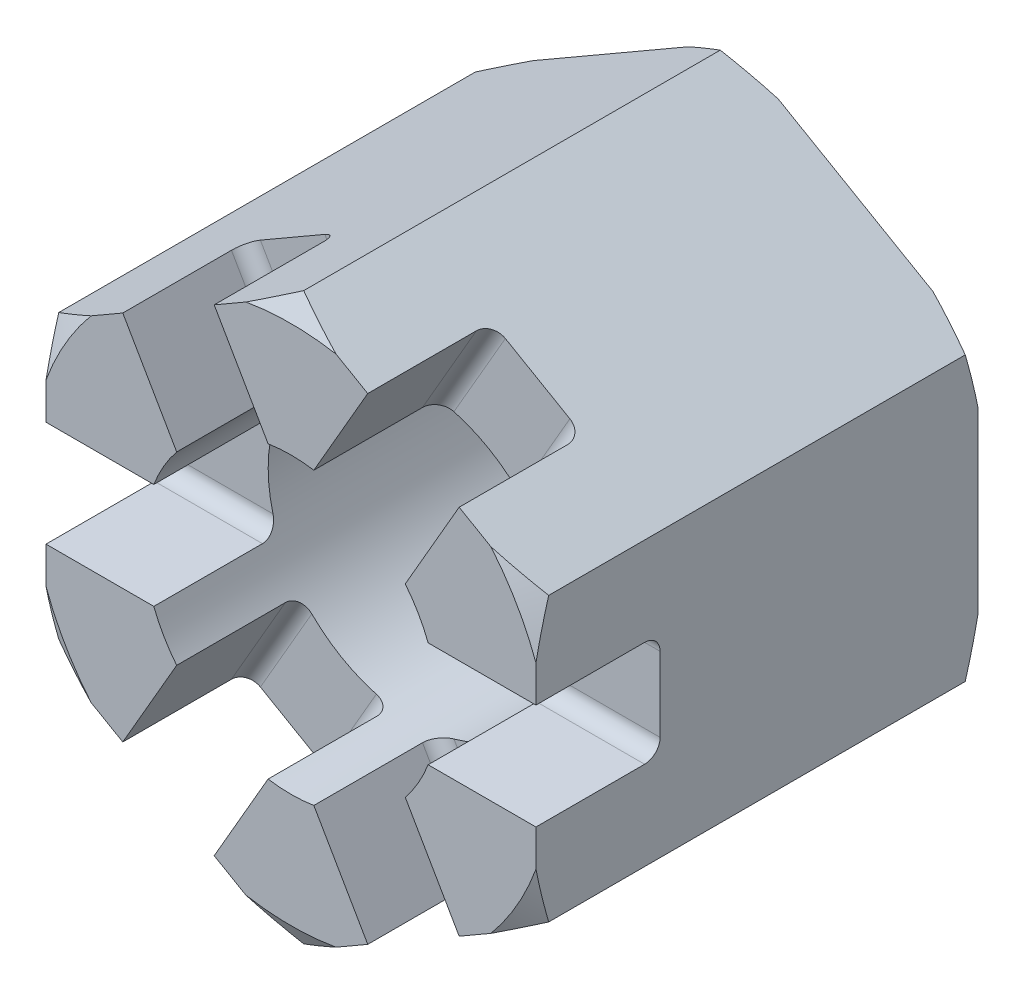
from build123d import *

# Parameters (mm, degrees)
SKETCH1_R          = 5.9175
BASE_EXTRUDE_DEPTH = 17.8
SKETCH2_OUTSIDE_W  = 112.978
SKETCH2_OUTSIDE_H  = 116.03
SKETCH2_OUTSIDE_R  = 10.5
CUT_EXTRUDE1_DEPTH = 24.321045753
CUT_EXTRUDE1_DRAFT = -60
SKETCH3_OUTSIDE_W  = 112.978
SKETCH3_OUTSIDE_H  = 116.03
SKETCH3_OUTSIDE_R  = 10.5
CUT_EXTRUDE2_DEPTH = 24.321045753
CUT_EXTRUDE2_DRAFT = -60
CUT_EXTRUDE3_DEPTH = 29.909659285
CIRPATTERN1_COUNT  = 3
CHAMFER1_SIZE      = 0.220833333


with BuildPart() as part:
    # Sketch1 → Base-Extrude (new body)
    with BuildSketch(Plane.XY):
        Polygon((0, 11.39), (-9.864029349, 5.695), (-9.864029349, -5.695), (0, -11.39), (9.864029349, -5.695), (9.864029349, 5.695), align=None)
        Circle(SKETCH1_R, mode=Mode.SUBTRACT)
    extrude(amount=BASE_EXTRUDE_DEPTH)


with BuildPart() as cut_extrude1_tool:
    # Sketch2 outside → Cut-Extrude1 (with draft: the straight prism first)
    with BuildSketch(Plane(origin=(0, 0, 0), x_dir=(-1, 0, 0), z_dir=(0, 0, -1))):
        Rectangle(SKETCH2_OUTSIDE_W, SKETCH2_OUTSIDE_H)
        Circle(SKETCH2_OUTSIDE_R, mode=Mode.SUBTRACT)
    extrude(amount=-CUT_EXTRUDE1_DEPTH)
    # Cut-Extrude1: the draft: its side faces are tilted about the plane it starts from
    cut_extrude1_sides = [cut_extrude1_tool.faces().sort_by_distance(p)[0] for p in [
        (0, -58.015, 12.160522876),
        (-56.489, 0, 12.160522876),
        (0, 58.015, 12.160522876),
        (56.489, 0, 12.160522876),
        (10.5, 0, 12.160522876),
    ]]
    draft(cut_extrude1_sides, Plane(origin=(0, 0, 0), x_dir=(-1, 0, 0), z_dir=(0, 0, -1)), CUT_EXTRUDE1_DRAFT)


with BuildPart() as part_1:
    add(part.part)

    # Cut-Extrude1: cut by cut_extrude1_tool
    add(cut_extrude1_tool.part, mode=Mode.SUBTRACT)


with BuildPart() as cut_extrude2_tool:
    # Sketch3 outside → Cut-Extrude2 (with draft: the straight prism first)
    with BuildSketch(Plane.XY.offset(17.8)):
        Rectangle(SKETCH3_OUTSIDE_W, SKETCH3_OUTSIDE_H)
        Circle(SKETCH3_OUTSIDE_R, mode=Mode.SUBTRACT)
    extrude(amount=-CUT_EXTRUDE2_DEPTH)
    # Cut-Extrude2: the draft: its side faces are tilted about the plane it starts from
    cut_extrude2_sides = [cut_extrude2_tool.faces().sort_by_distance(p)[0] for p in [
        (0, -58.015, 5.639477124),
        (56.489, 0, 5.639477124),
        (0, 58.015, 5.639477124),
        (-56.489, 0, 5.639477124),
        (-10.5, 0, 5.639477124),
    ]]
    draft(cut_extrude2_sides, Plane.XY.offset(17.8), CUT_EXTRUDE2_DRAFT)


with BuildPart() as part_2:
    add(part_1.part)

    # Cut-Extrude2: cut by cut_extrude2_tool
    add(cut_extrude2_tool.part, mode=Mode.SUBTRACT)

    # Sketch6 → Cut-Extrude3 (cut, through all)
    with BuildSketch(Plane(origin=(9.864029349, 0, 0), x_dir=(0, 0, -1), z_dir=(1, 0, 0))):
        with BuildLine():
            Line((-17.8, -2.125), (-17.8, 2.125))
            Line((-17.8, 2.125), (-13.425, 2.125))
            ThreePointArc((-13.425, 2.125), (-12.983058262, 1.941941738), (-12.8, 1.5))
            Line((-12.8, 1.5), (-12.8, -1.5))
            ThreePointArc((-12.8, -1.5), (-12.983058262, -1.941941738), (-13.425, -2.125))
            Line((-13.425, -2.125), (-17.8, -2.125))
        make_face()
    cut_extrude3 = extrude(amount=-CUT_EXTRUDE3_DEPTH, mode=Mode.SUBTRACT)

    # CirPattern1: Cut-Extrude3 ×3 about axis
    cirpattern1_axis = Axis((0, 0, 0), (0, 0, 1))
    for i in range(1, CIRPATTERN1_COUNT):
        add(cut_extrude3.rotate(cirpattern1_axis, i * 360 / CIRPATTERN1_COUNT), mode=Mode.SUBTRACT)

    # Chamfer1
    chamfer1_edges = [part_2.edges().sort_by_distance(p)[0] for p in [
        (-5.9175, 0, 0),
    ]]
    chamfer(chamfer1_edges, length=CHAMFER1_SIZE)


solid = part_2.part
